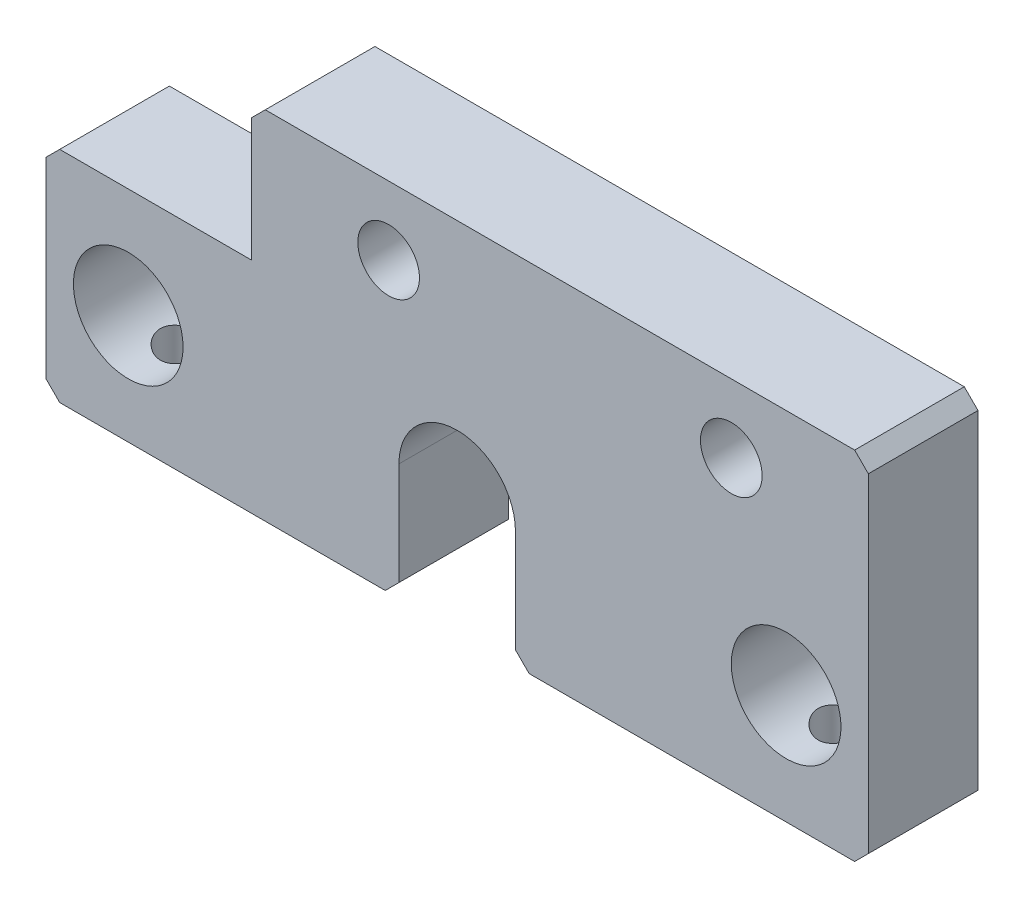
from build123d import *

# Parameters (mm, degrees)
SKETCH1_W              = 60
SKETCH1_H              = 26
SKETCH1_R              = 4
BOSS_EXTRUDE1_DEPTH    = 8
CUT_EXTRUDE1_DEPTH     = 41.496913463
M4_TAPPED_HOLE1_REACH  = 42.497
M4_TAPPED_HOLE1_BORE_R = 1.65
SKETCH8_W              = 15
SKETCH8_H              = 10
CUT_EXTRUDE2_DEPTH     = 41.496913482
SKETCH9_R              = 2.25
CUT_EXTRUDE3_DEPTH     = 41.496913482
CHAMFER1_SIZE          = 1


with BuildPart() as part:
    # Sketch1 → Boss-Extrude1 (new body)
    with BuildSketch(Plane.XY):
        with Locations((0, 13)):
            Rectangle(SKETCH1_W, SKETCH1_H)
        with Locations((-24, 8)):
            Circle(SKETCH1_R, mode=Mode.SUBTRACT)
        with Locations(Location((24, 8, 0), (0, 0, 180))):
            Circle(SKETCH1_R, mode=Mode.SUBTRACT)
    extrude(amount=BOSS_EXTRUDE1_DEPTH)

    # Sketch2 → Cut-Extrude1 (cut, through all)
    with BuildSketch(Plane.XY.offset(8)):
        with BuildLine():
            Line((-4.25, 0), (-4.25, 8.5))
            ThreePointArc((-4.25, 8.5), (0, 12.75), (4.25, 8.5))
            Line((4.25, 8.5), (4.25, 0))
            ThreePointArc((4.25, 0), (0, -4.25), (-4.25, 0))
        make_face()
    extrude(amount=-CUT_EXTRUDE1_DEPTH, mode=Mode.SUBTRACT)

    # M4 Tapped Hole1 bore → M4 Tapped Hole1 (cut, up to next)
    with BuildSketch(Plane.XZ, mode=Mode.PRIVATE) as m4_tapped_hole1_sk1:
        with Locations((-24, 4)):
            Circle(M4_TAPPED_HOLE1_BORE_R)
    m4_tapped_hole1_tool1 = extrude(m4_tapped_hole1_sk1.sketch, amount=-M4_TAPPED_HOLE1_REACH, mode=Mode.PRIVATE) & part.part
    # M4 Tapped Hole1 bore → M4 Tapped Hole1 (cut, up to next)
    with BuildSketch(Plane.XZ, mode=Mode.PRIVATE) as m4_tapped_hole1_sk2:
        with Locations((24, 4)):
            Circle(M4_TAPPED_HOLE1_BORE_R)
    m4_tapped_hole1_tool2 = extrude(m4_tapped_hole1_sk2.sketch, amount=-M4_TAPPED_HOLE1_REACH, mode=Mode.PRIVATE) & part.part
    add(m4_tapped_hole1_tool1.solids().sort_by_distance((-24, 0, 4))[0], mode=Mode.SUBTRACT)
    add(m4_tapped_hole1_tool2.solids().sort_by_distance((24, 0, 4))[0], mode=Mode.SUBTRACT)

    # Sketch8 → Cut-Extrude2 (cut, through all)
    with BuildSketch(Plane(origin=(0, 0, 0), x_dir=(-1, 0, 0), z_dir=(0, 0, -1))):
        with Locations((22.5, 21)):
            Rectangle(SKETCH8_W, SKETCH8_H)
    extrude(amount=-CUT_EXTRUDE2_DEPTH, mode=Mode.SUBTRACT)

    # Sketch9 → Cut-Extrude3 (cut, through all)
    with BuildSketch(Plane(origin=(0, 0, 0), x_dir=(-1, 0, 0), z_dir=(0, 0, -1))):
        with Locations((-20, 21)):
            Circle(SKETCH9_R)
        with Locations((5, 21)):
            Circle(SKETCH9_R)
    extrude(amount=-CUT_EXTRUDE3_DEPTH, mode=Mode.SUBTRACT)

    # Chamfer1
    chamfer1_edges = [part.edges().sort_by_distance(p)[0] for p in [
        (4.25, 0, 4),
        (-4.25, 0, 4),
        (-15, 26, 4),
        (-30, 16, 4),
        (30, 0, 4),
        (-30, 0, 4),
        (30, 26, 4),
    ]]
    chamfer(chamfer1_edges, length=CHAMFER1_SIZE)


solid = part.part
